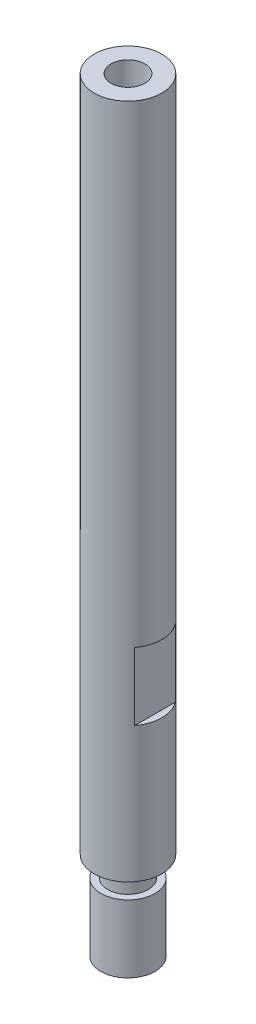
SolidWorks part; units mm, degrees
ref_plane "Front Plane" through (0, 0, 0) normal (0, 0, 1) x (1, 0, 0)
ref_plane "Top Plane" through (0, 0, 0) normal (0, 1, 0) x (1, 0, 0)
ref_plane "Right Plane" through (0, 0, 0) normal (1, 0, 0) x (0, 0, -1)
sketch "Sketch1" plane through (0, 0, 0) normal (0, 0, 1) x (1, 0, 0)
  line L0 (0, 14.171) -> (0, -98.829)
  line L1 (0, -98.829) -> (-4, -98.829)
  line L2 (-4, -98.829) -> (-4, -88.829)
  line L3 (-4, -88.829) -> (-3, -88.829)
  line L4 (-3, -88.829) -> (-3, -85.829)
  line L5 (-3, -85.829) -> (-5, -85.829)
  line L6 (-5, -85.829) -> (-5, 14.171)
  line L7 (-5, 14.171) -> (0, 14.171)
  dimension "D1" = 5
  dimension "D2" = 100
  dimension "D3" = 3
  dimension "D4" = 113
  dimension "D5" = 4
  dimension "D6" = 3
revolve "Revolve1" add sketch "Sketch1" angle 360 about L0
cosmetic thread "Cosmetic Thread1" parameters "D2"=6.647
sketch "Sketch2" plane through (0, 0, 0) normal (0, 0, 1) x (1, 0, 0)
  line L0 (-5, 14.171) -> (-5, -85.829) construction
  line L1 (-5, -55.829) -> (-4, -55.829)
  line L2 (-5, -55.829) -> (-5, -65.829)
  line L3 (-5, -65.829) -> (-4, -65.829)
  line L4 (-4, -55.829) -> (-4, -65.829)
  line L5 (5, 14.171) -> (-5, 14.171) construction
  line L6 (0, -85.829) -> (0, -35.6063) construction
  line L7 (-3, -85.829) -> (3, -85.829) construction
  line L8 (4, -55.829) -> (4, -65.829)
  line L9 (5, -65.829) -> (4, -65.829)
  line L10 (5, -55.829) -> (5, -65.829)
  line L11 (5, -55.829) -> (4, -55.829)
  point P6 (-4.5, -55.829)
  dimension "D1" = 1
  dimension "D2" = 10
  dimension "D3" = 70
extrude "Cut-Extrude1" cut sketch "Sketch2" against normal through all both and the other way through all
hole_wizard "M6 Tapped Hole1" positions "Sketch3" profile "Sketch4" tap size "M6" standard "GB"
sketch "Sketch3" plane through (0, 14.171, 0) normal (0, 1, 0) x (1, 0, 0)
  point P0 (0, 0)
sketch "Sketch4" plane through (0, 14.171, 0) normal (1, 0, 0) x (0, 0, 1)
  line L0 (0, 0) -> (0, 13.5022)
  line L1 (0, 13.5022) -> (2.5, 12)
  line L2 (2.5, 12) -> (2.5, 0)
  line L5 (2.5, 0) -> (0, 0)
  line L10 (0, 13.5022) -> (-2.5, 12) construction
  line L11 (0, -6.35) -> (0, 107.95) construction
  dimension "螺纹孔钻头直径" = 5
  dimension "螺纹孔钻头深度" = 12
  dimension "导头角度" = 118
cosmetic thread "孔螺蚊线1" parameters "D1"=8, "D2"=6
